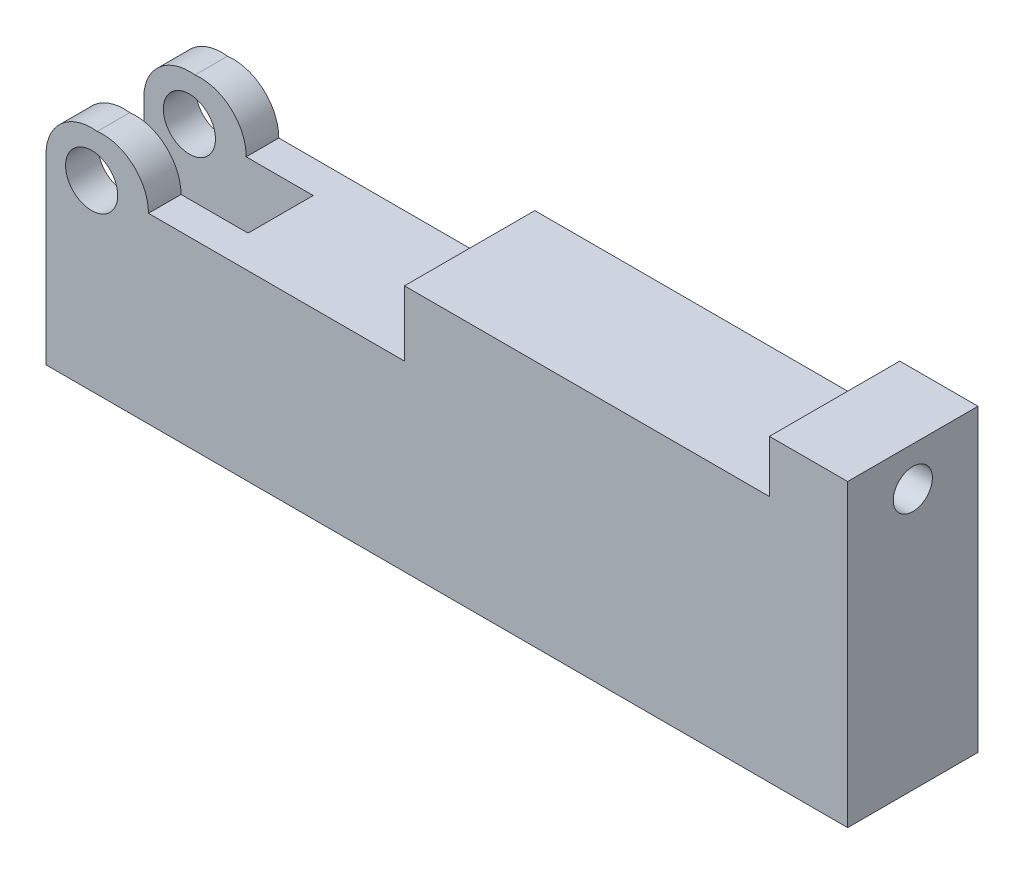
from build123d import *

# Parameters (mm, degrees)
SKETCH_1_R          = 2
EXTRUDE_1_DEPTH     = 10
SKETCH_2_R          = 1.5
CUT_EXTRUDE_1_DEPTH = 6
SKETCH_3_W          = 5
SKETCH_3_H          = 9
CUT_EXTRUDE_2_DEPTH = 13


with BuildPart() as part:
    # 草图1 → 凸台-拉伸1 (new body)
    with BuildSketch(Plane.XY):
        with BuildLine():
            Line((-46.664590164, 1.25102459), (-27.024590164, 1.25102459))
            Line((-27.024590164, 1.25102459), (-27.024590164, 6.25102459))
            Line((-27.024590164, 6.25102459), (0.975409836, 6.25102459))
            Line((0.975409836, 6.25102459), (0.975409836, 10.25102459))
            Line((0.975409836, 10.25102459), (6.975409836, 10.25102459))
            Line((6.975409836, 10.25102459), (6.975409836, -12.74897541))
            Line((6.975409836, -12.74897541), (-54.524590164, -12.74897541))
            Line((-54.524590164, -12.74897541), (-54.524590164, 1.25102459))
            ThreePointArc((-54.524590164, 1.25102459), (-53.342455561, 3.873523399), (-50.594590164, 4.724509872))
            ThreePointArc((-50.594590164, 4.724509872), (-47.846724767, 3.873523399), (-46.664590164, 1.25102459))
        make_face()
        with Locations((-51.024590164, 1.25102459)):
            Circle(SKETCH_1_R, mode=Mode.SUBTRACT)
    extrude(amount=EXTRUDE_1_DEPTH)

    # 草图2 → 切除-拉伸1 (cut)
    with BuildSketch(Plane(origin=(6.975409836, 0, 0), x_dir=(0, 0, -1), z_dir=(1, 0, 0))):
        with Locations((-5, 7.25102459)):
            Circle(SKETCH_2_R)
    extrude(amount=-CUT_EXTRUDE_1_DEPTH, mode=Mode.SUBTRACT)

    # 草图3 → 切除-拉伸2 (cut)
    with BuildSketch(Plane.ZY.offset(54.524590164)):
        with Locations((5, 0.25102459)):
            Rectangle(SKETCH_3_W, SKETCH_3_H)
    extrude(amount=-CUT_EXTRUDE_2_DEPTH, mode=Mode.SUBTRACT)


solid = part.part
